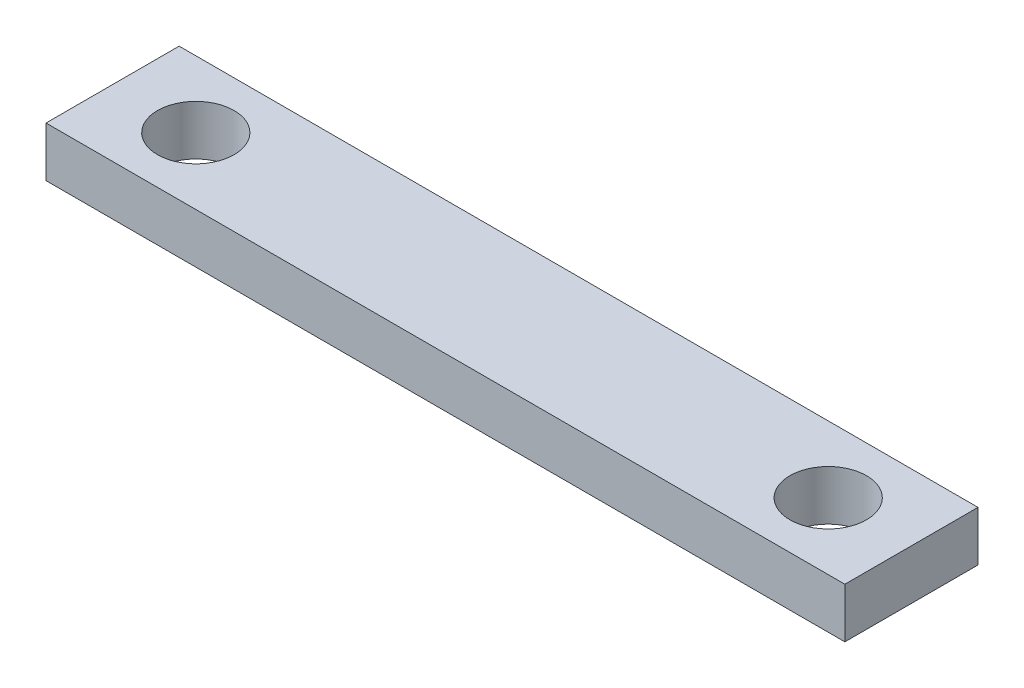
from build123d import *

# Parameters (mm, degrees)
SKETCH1_W                  = 24
SKETCH1_H                  = 4
BOSS_EXTRUDE1_DEPTH        = 0.75
F_2_3_2_3_DIAMETER_HOLE1_D = 2.3


with BuildPart() as part:
    # Sketch1 → Boss-Extrude1 (new, symmetric)
    with BuildSketch(Plane(origin=(0, 0, 0), x_dir=(1, 0, 0), z_dir=(0, 1, 0))):
        Rectangle(SKETCH1_W, SKETCH1_H)
    extrude(amount=BOSS_EXTRUDE1_DEPTH, both=True)

    # Ø2.3 (2.3) Diameter Hole1 (through all)
    with Locations(Plane(origin=(0, 0.75, 0), x_dir=(1, 0, 0), z_dir=(0, 1, 0))):
        with Locations((-9.5, 0), (9.5, 0)):
            Hole(F_2_3_2_3_DIAMETER_HOLE1_D / 2)


solid = part.part
